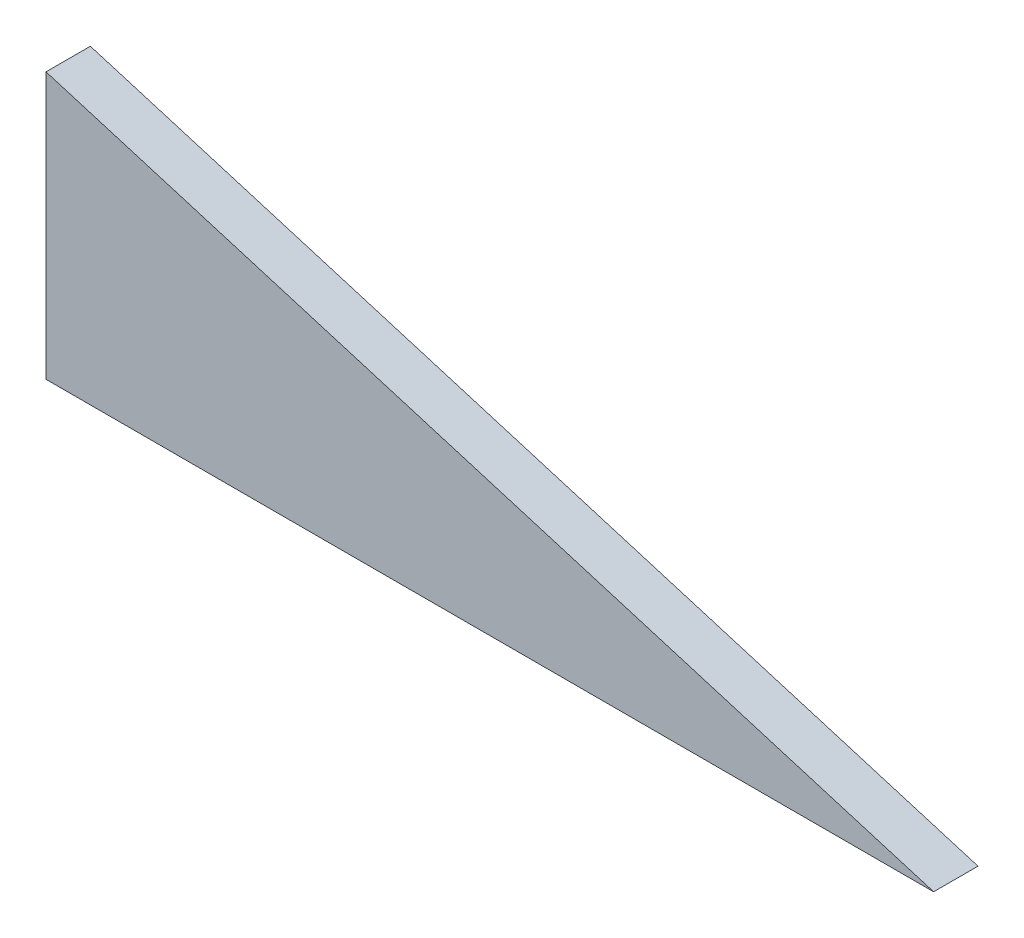
SolidWorks part; units mm, degrees
ref_plane "前视基准面" through (0, 0, 0) normal (0, 0, 1) x (1, 0, 0)
ref_plane "上视基准面" through (0, 0, 0) normal (0, 1, 0) x (1, 0, 0)
ref_plane "右视基准面" through (0, 0, 0) normal (1, 0, 0) x (0, 0, -1)
sketch "草图1" plane through (0, 0, 0) normal (0, 0, 1) x (1, 0, 0)
  line L0 (0, 0) -> (0, 30)
  line L3 (0, 0) -> (100, 0)
  line L4 (100, 0) -> (0, 30)
extrude "凸台-拉伸1" add sketch "草图1" along normal blind 5
